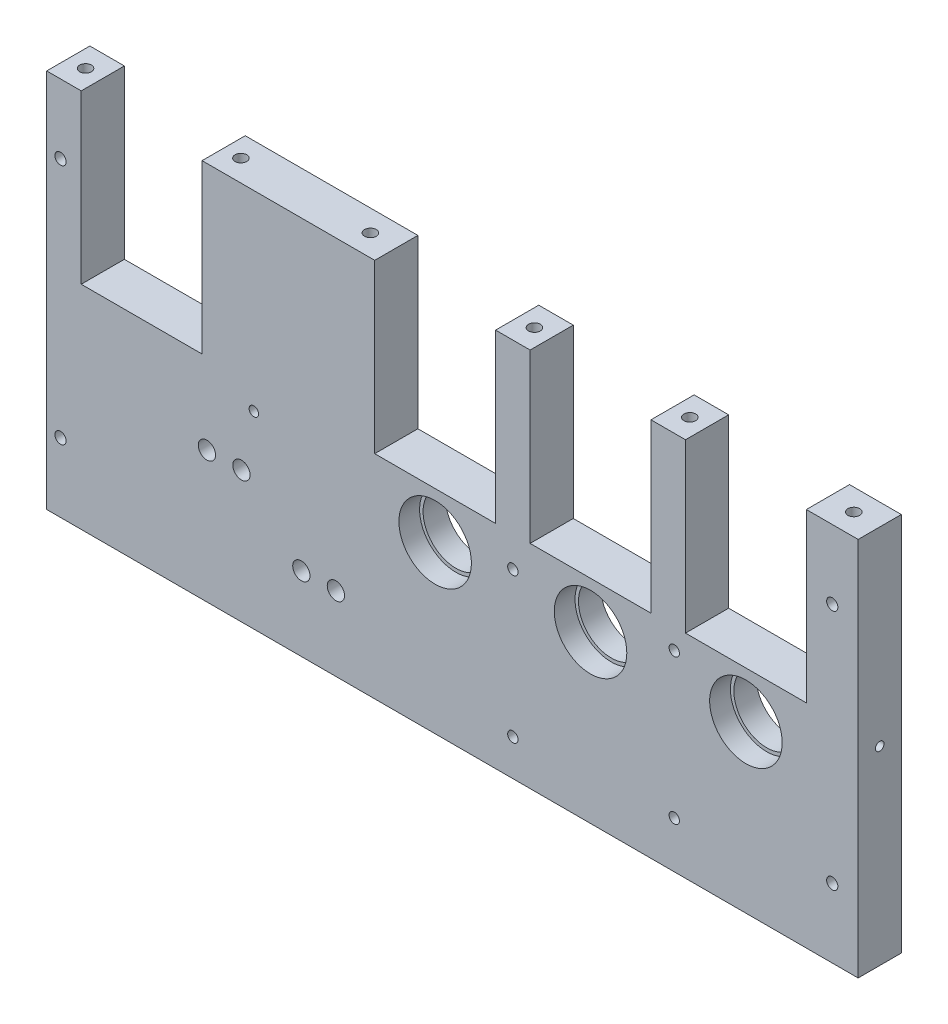
from build123d import *

# Parameters (mm, degrees)
SKETCH1_W                       = 470
SKETCH1_H                       = 260
BOSS_EXTRUDE1_DEPTH             = 12.5
SKETCH4_W                       = 70
SKETCH4_H                       = 97
CUT_EXTRUDE3_DEPTH              = 97
SKETCH8_W                       = 627.570760349
SKETCH8_H                       = 104.374926458
CUT_EXTRUDE7_DEPTH              = 40
M8_TAPPED_HOLE1_D               = 6.8
M8_TAPPED_HOLE1_DEPTH           = 20
M8_TAPPED_HOLE1_TIP             = 2.042926105
M10_TAPPED_HOLE1_D              = 8.5
M10_TAPPED_HOLE1_DEPTH          = 27.5
M10_TAPPED_HOLE1_TIP            = 2.553657631
SKETCH17_R                      = 19
CUT_EXTRUDE10_DEPTH             = 270.722079185
SKETCH18_R                      = 21
CUT_EXTRUDE11_DEPTH             = 12
SKETCH22_R                      = 3
CUT_EXTRUDE13_DEPTH             = 270.722079185
SKETCH23_R                      = 3.25
CUT_EXTRUDE14_DEPTH             = 270.722079185
SKETCH24_R                      = 5.5
CUT_EXTRUDE15_DEPTH             = 10
LPATTERN1_COUNT                 = 2
LPATTERN1_PITCH                 = 447
SKETCH26_R                      = 2.75
CUT_EXTRUDE17_DEPTH             = 270.722079185
SKETCH27_R                      = 5
CUT_EXTRUDE18_DEPTH             = 8
SKETCH28_R                      = 5
CUT_EXTRUDE19_DEPTH             = 30
M6_TAPPED_HOLE1_D               = 5
M6_TAPPED_HOLE1_DEPTH           = 15
M6_TAPPED_HOLE1_TIP             = 1.502151548
M6_TAPPED_HOLE1_ON_FACE_2_D     = 5
M6_TAPPED_HOLE1_ON_FACE_2_DEPTH = 15
M6_TAPPED_HOLE1_ON_FACE_2_TIP   = 1.502151548


with BuildPart() as part:
    # Sketch1 → Boss-Extrude1 (new, symmetric)
    with BuildSketch(Plane.XY):
        Rectangle(SKETCH1_W, SKETCH1_H)
    extrude(amount=BOSS_EXTRUDE1_DEPTH, both=True)

    # Sketch4 → Cut-Extrude3 (cut)
    with BuildSketch(Plane.XY.offset(12.5)):
        with Locations((-180, 81.5)):
            Rectangle(SKETCH4_W, SKETCH4_H)
        with Locations((-10, 81.5)):
            Rectangle(SKETCH4_W, SKETCH4_H)
        with Locations((80, 81.5)):
            Rectangle(SKETCH4_W, SKETCH4_H)
        with Locations((170, 81.5)):
            Rectangle(SKETCH4_W, SKETCH4_H)
    extrude(amount=-CUT_EXTRUDE3_DEPTH, mode=Mode.SUBTRACT)

    # Sketch8 → Cut-Extrude7 (cut)
    with BuildSketch(Plane.XY.offset(12.5)):
        with Locations((-4.378447024, -142.187463229)):
            Rectangle(SKETCH8_W, SKETCH8_H)
    extrude(amount=-CUT_EXTRUDE7_DEPTH, mode=Mode.SUBTRACT)

    # M8 Tapped Hole1
    with Locations(Plane(origin=(0, 130, 0), x_dir=(1, 0, 0), z_dir=(0, 1, 0))):
        with Locations((-225, 0), (-135, 0), (35, 0), (125, 0), (220, 0), (-60, 0)):
            Hole(M8_TAPPED_HOLE1_D / 2, depth=M8_TAPPED_HOLE1_DEPTH)
            with Locations((0, 0, -(M8_TAPPED_HOLE1_DEPTH + M8_TAPPED_HOLE1_TIP / 2))):  # 118° drill point
                Cone(0, M8_TAPPED_HOLE1_D / 2, M8_TAPPED_HOLE1_TIP, mode=Mode.SUBTRACT)

    # M10 Tapped Hole1
    with Locations(Plane(origin=(0, -90, 0), x_dir=(-1, 0, 0), z_dir=(0, -1, 0))):
        with Locations((-155, 0), (155, 0)):
            Hole(M10_TAPPED_HOLE1_D / 2, depth=M10_TAPPED_HOLE1_DEPTH)
            with Locations((0, 0, -(M10_TAPPED_HOLE1_DEPTH + M10_TAPPED_HOLE1_TIP / 2))):  # 118° drill point
                Cone(0, M10_TAPPED_HOLE1_D / 2, M10_TAPPED_HOLE1_TIP, mode=Mode.SUBTRACT)

    # Sketch17 → Cut-Extrude10 (cut, through all)
    with BuildSketch(Plane.XY.offset(12.5)):
        with Locations((170, 6)):
            Circle(SKETCH17_R)
        with Locations((80, 6)):
            Circle(SKETCH17_R)
        with Locations((-10, 6)):
            Circle(SKETCH17_R)
    extrude(amount=-CUT_EXTRUDE10_DEPTH, mode=Mode.SUBTRACT)

    # Sketch18 → Cut-Extrude11 (cut)
    with BuildSketch(Plane.XY.offset(12.5)):
        with Locations((170, 6)):
            Circle(SKETCH18_R)
        with Locations((80, 6)):
            Circle(SKETCH18_R)
        with Locations((-10, 6)):
            Circle(SKETCH18_R)
    extrude(amount=-CUT_EXTRUDE11_DEPTH, mode=Mode.SUBTRACT)

    # Sketch22 → Cut-Extrude13 (cut, through all)
    with BuildSketch(Plane(origin=(0, 0, -12.5), x_dir=(-1, 0, 0), z_dir=(0, 0, -1))):
        with Locations((-128.5, 21)):
            Circle(SKETCH22_R)
        with Locations((-128.5, -63)):
            Circle(SKETCH22_R)
        with Locations((-35, 15)):
            Circle(SKETCH22_R)
        with Locations((-35, -69)):
            Circle(SKETCH22_R)
    extrude(amount=-CUT_EXTRUDE13_DEPTH, mode=Mode.SUBTRACT)

    # Sketch23 → Cut-Extrude14 (cut, through all)
    with BuildSketch(Plane(origin=(0, 0, -12.5), x_dir=(-1, 0, 0), z_dir=(0, 0, -1))):
        with Locations((-220, 90)):
            Circle(SKETCH23_R)
        with Locations((-220, -50)):
            Circle(SKETCH23_R)
    cut_extrude14 = extrude(amount=-CUT_EXTRUDE14_DEPTH, mode=Mode.SUBTRACT)

    # Sketch24 → Cut-Extrude15 (cut)
    with BuildSketch(Plane(origin=(0, 0, -12.5), x_dir=(-1, 0, 0), z_dir=(0, 0, -1))):
        with Locations((-220, 90)):
            Circle(SKETCH24_R)
        with Locations((-220, -50)):
            Circle(SKETCH24_R)
    cut_extrude15 = extrude(amount=-CUT_EXTRUDE15_DEPTH, mode=Mode.SUBTRACT)

    # LPattern1: Cut-Extrude14, Cut-Extrude15 ×2
    with Locations(*[(-i * LPATTERN1_PITCH, 0, 0) for i in range(1, LPATTERN1_COUNT)]):
        add(cut_extrude14, mode=Mode.SUBTRACT)
        add(cut_extrude15, mode=Mode.SUBTRACT)

    # Sketch26 → Cut-Extrude17 (cut, through all)
    with BuildSketch(Plane(origin=(0, 0, -12.5), x_dir=(-1, 0, 0), z_dir=(0, 0, -1))):
        with Locations((115, 19.25)):
            Circle(SKETCH26_R)
    extrude(amount=-CUT_EXTRUDE17_DEPTH, mode=Mode.SUBTRACT)

    # Sketch27 → Cut-Extrude18 (cut)
    with BuildSketch(Plane(origin=(0, 0, -12.5), x_dir=(-1, 0, 0), z_dir=(0, 0, -1))):
        with Locations((115, 19.25)):
            Circle(SKETCH27_R)
    extrude(amount=-CUT_EXTRUDE18_DEPTH, mode=Mode.SUBTRACT)

    # Sketch28 → Cut-Extrude19 (cut)
    with BuildSketch(Plane(origin=(0, 0, -12.5), x_dir=(-1, 0, 0), z_dir=(0, 0, -1))):
        with Locations((67.5, -47)):
            Circle(SKETCH28_R)
        with Locations((87.5, -47)):
            Circle(SKETCH28_R)
        with Locations((122.2, -13.8)):
            Circle(SKETCH28_R)
        with Locations((142.2, -13.8)):
            Circle(SKETCH28_R)
    extrude(amount=-CUT_EXTRUDE19_DEPTH, mode=Mode.SUBTRACT)

    # M6 Tapped Hole1
    with Locations(Plane(origin=(-235, 20, 0), x_dir=(0, 0, -1), z_dir=(-1, 0, 0))):
        with Locations((0, 0)):
            Hole(M6_TAPPED_HOLE1_D / 2, depth=M6_TAPPED_HOLE1_DEPTH)
            with Locations((0, 0, -(M6_TAPPED_HOLE1_DEPTH + M6_TAPPED_HOLE1_TIP / 2))):  # 118° drill point
                Cone(0, M6_TAPPED_HOLE1_D / 2, M6_TAPPED_HOLE1_TIP, mode=Mode.SUBTRACT)

    # M6 Tapped Hole1 on face 2
    with Locations(Plane(origin=(235, 20, 0), x_dir=(0, 0, 1), z_dir=(1, 0, 0))):
        with Locations((0, 0)):
            Hole(M6_TAPPED_HOLE1_ON_FACE_2_D / 2, depth=M6_TAPPED_HOLE1_ON_FACE_2_DEPTH)
            with Locations((0, 0, -(M6_TAPPED_HOLE1_ON_FACE_2_DEPTH + M6_TAPPED_HOLE1_ON_FACE_2_TIP / 2))):  # 118° drill point
                Cone(0, M6_TAPPED_HOLE1_ON_FACE_2_D / 2, M6_TAPPED_HOLE1_ON_FACE_2_TIP, mode=Mode.SUBTRACT)


solid = part.part
